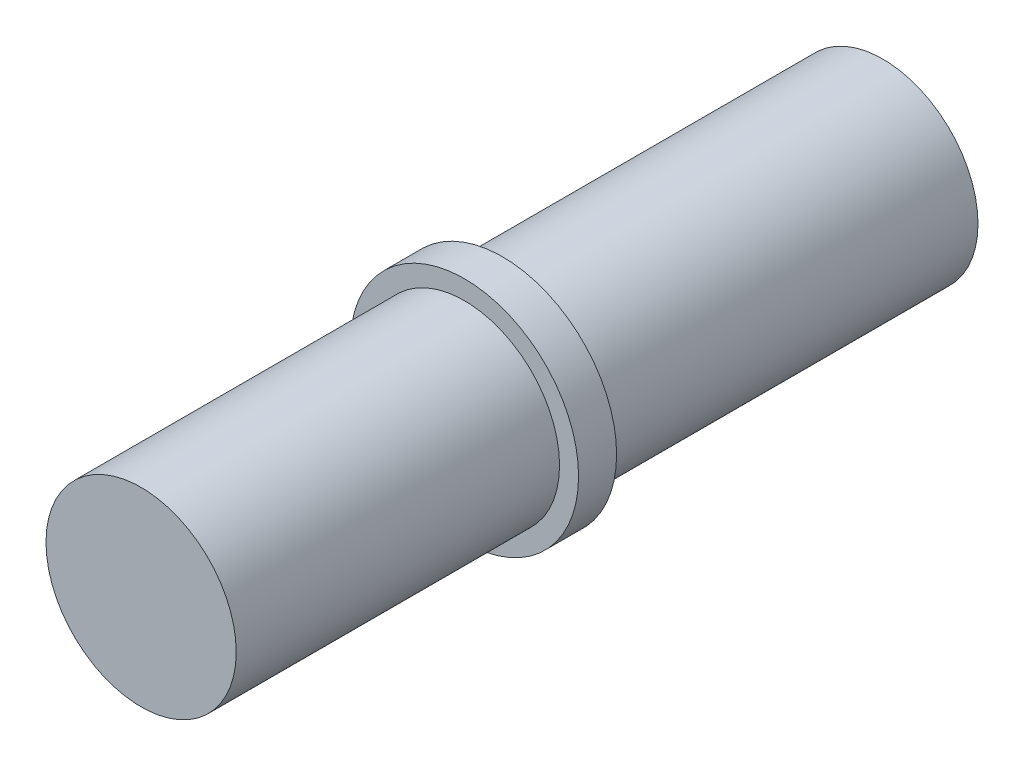
from build123d import *

# Parameters (mm, degrees)
SKETCH_1_R          = 7.5
EXTRUDE_1_DEPTH     = 100
EXTRUDE_START       = -25.5
SKETCH_2_R          = 9
EXTRUDE_2_DEPTH     = 3
EXTRUDE_START_2     = -28.5
SKETCH_3_R          = 9
EXTRUDE_3_DEPTH     = 3
EXTRUDE_START_3     = 40
SKETCH_4_R          = 7.5
EXTRUDE_4_DEPTH     = 40
SKETCH_5_R          = 10
CUT_EXTRUDE_2_DEPTH = 81.5


with BuildPart() as part:
    # 草图1 → 凸台-拉伸1 (new body)
    with BuildSketch(Plane.XY):
        Circle(SKETCH_1_R)
    extrude(amount=EXTRUDE_1_DEPTH)

    # 草图2 → 凸台-拉伸2 (add)
    with BuildSketch(Plane.XY.offset(100).offset(EXTRUDE_START)):
        Circle(SKETCH_2_R)
    extrude(amount=-EXTRUDE_2_DEPTH)

    # 草图3 → 凸台-拉伸3 (add)
    with BuildSketch(Plane(origin=(0, 0, 0), x_dir=(-1, 0, 0), z_dir=(0, 0, -1)).offset(EXTRUDE_START_2)):
        with Locations(Location((0, 0, 0), (0, 0, 180))):
            Circle(SKETCH_3_R)
    extrude(amount=EXTRUDE_3_DEPTH)

    # 草图4 → 凸台-拉伸4 (add)
    with BuildSketch(Plane(origin=(0, 0, 0), x_dir=(-1, 0, 0), z_dir=(0, 0, -1)).offset(EXTRUDE_START_3)):
        Circle(SKETCH_4_R)
    extrude(amount=-EXTRUDE_4_DEPTH)

    # 草图5 → 切除-拉伸2 (cut)
    with BuildSketch(Plane(origin=(0, 0, -40), x_dir=(-1, 0, 0), z_dir=(0, 0, -1))):
        Circle(SKETCH_5_R)
    extrude(amount=-CUT_EXTRUDE_2_DEPTH, mode=Mode.SUBTRACT)


solid = part.part
